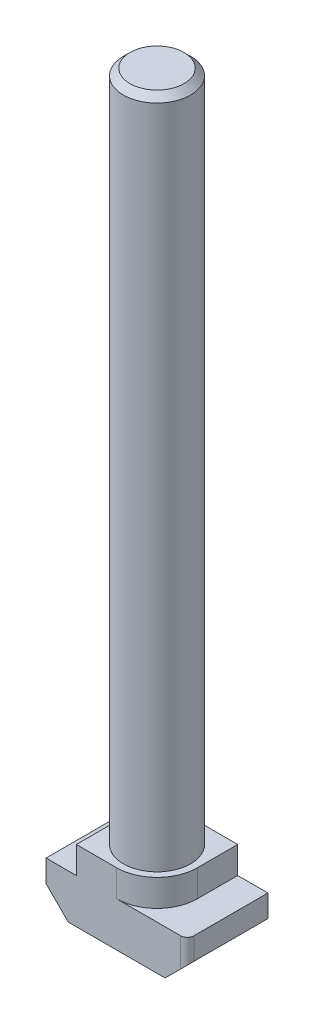
from build123d import *

# Parameters (mm, degrees)
BOSS_EXTRUDE1_DEPTH = 6
SKETCH2_W           = 2.25
SKETCH2_H           = 2
CUT_EXTRUDE1_DEPTH  = 9.628586211
SKETCH3_W           = 2.25
SKETCH3_H           = 2
CUT_EXTRUDE2_DEPTH  = 9.628586211
SKETCH4_W           = 2.5
SKETCH4_H           = 50
CHAMFER1_SIZE       = 0.4905
FILLET1_R           = 0.5
FILLET2_R           = 3


with BuildPart() as part:
    # Sketch1 → Boss-Extrude1 (new body)
    with BuildSketch(Plane(origin=(0, 0, -3), x_dir=(-1, 0, 0), z_dir=(0, 0, -1))):
        Polygon((5.25, 2), (-5.25, 2), (-5.25, -1.65), (-3.6, -3.3), (3.6, -3.3), (5.25, -1.65), align=None)
    extrude(amount=-BOSS_EXTRUDE1_DEPTH)

    # Sketch2 → Cut-Extrude1 (cut, through all)
    with BuildSketch(Plane.XY.offset(3)):
        with Locations((-4.125, 1)):
            Rectangle(SKETCH2_W, SKETCH2_H)
    extrude(amount=-CUT_EXTRUDE1_DEPTH, mode=Mode.SUBTRACT)

    # Sketch3 → Cut-Extrude2 (cut, through all)
    with BuildSketch(Plane.XY.offset(3)):
        with Locations((4.125, 1)):
            Rectangle(SKETCH3_W, SKETCH3_H)
    extrude(amount=-CUT_EXTRUDE2_DEPTH, mode=Mode.SUBTRACT)

    # Sketch4 → Revolve1 (revolve)
    with BuildSketch(Plane(origin=(0, 0, 0), x_dir=(-1, 0, 0), z_dir=(0, 0, -1)), mode=Mode.PRIVATE) as revolve1_sk:
        with Locations((-1.25, 27)):
            Rectangle(SKETCH4_W, SKETCH4_H)
    revolve(revolve1_sk.sketch.rotate(Axis((0, 2, 0), (0, 1, 0)), 180), axis=Axis((0, 2, 0), (0, 1, 0)))

    # Chamfer1
    chamfer1_edges = [part.edges().sort_by_distance(p)[0] for p in [
        (2.5, 52, 0),
    ]]
    chamfer(chamfer1_edges, length=CHAMFER1_SIZE)

    # Fillet1
    fillet1_edges = [part.edges().sort_by_distance(p)[0] for p in [
        (5.25, -0.825, 3),
        (-5.25, -0.825, -3),
    ]]
    fillet(fillet1_edges, radius=FILLET1_R)

    # Fillet2
    fillet2_edges = [part.edges().sort_by_distance(p)[0] for p in [
        (-3, 1, -3),
        (3, 1, 3),
    ]]
    fillet(fillet2_edges, radius=FILLET2_R)


solid = part.part
